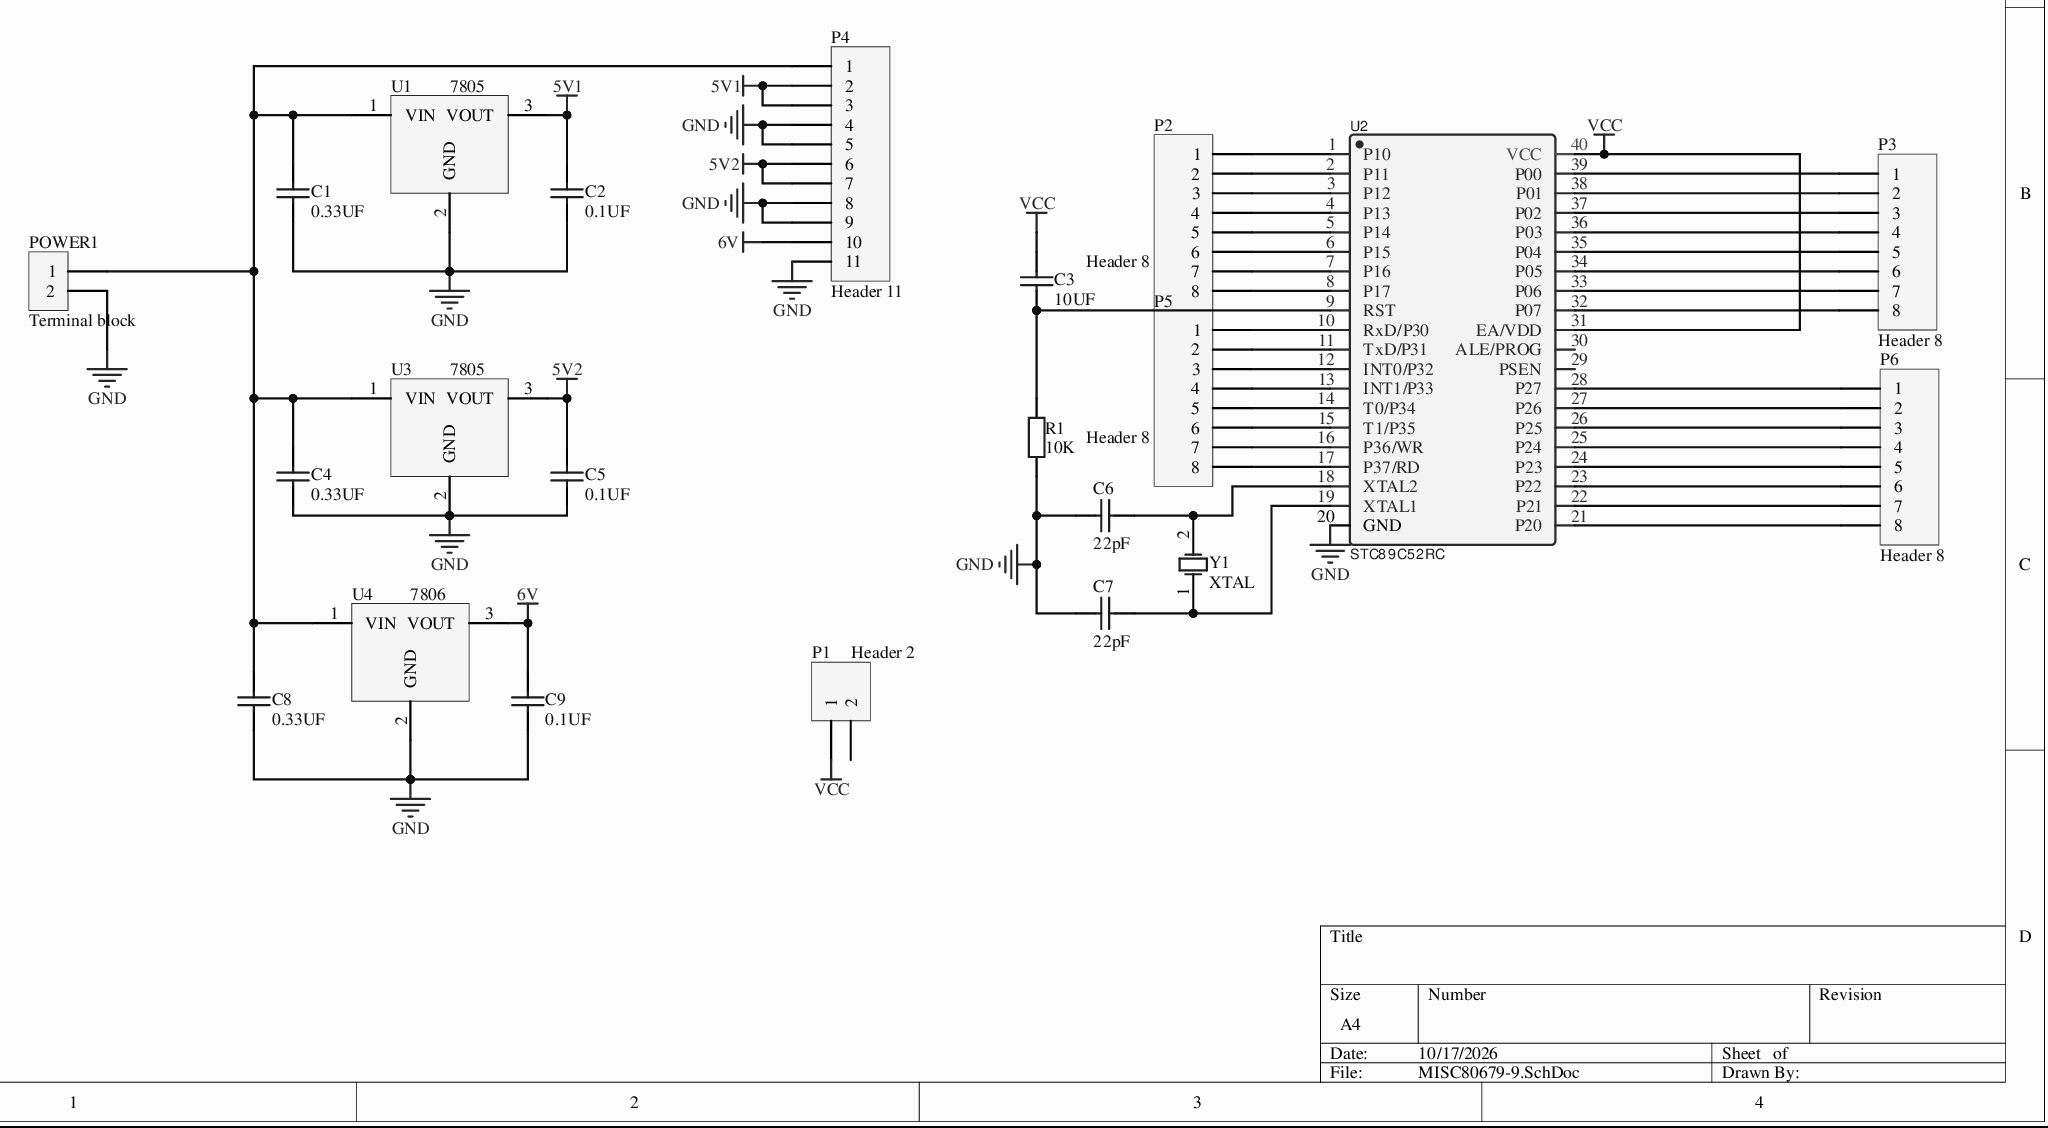
[diagram p0: MISC80679-9.SchDoc]
# Altium project MISC80679-3.PrjPcb
1 sheet, 22 parts. Net scope: global (net labels, ports and power ports of the same name join across sheets).
Board file: MISC80679.PcbDoc

## Sheet MISC80679-9.SchDoc
size A4

### Parts
C1  0.33UF  [CC 1.8*3.6]
C2  0.1UF  [CC 1.8*3.6]
C3  10UF  [CAP 1.5*4*8]
C4  0.33UF  [CC 1.8*3.6]
C5  0.1UF  [CC 1.8*3.6]
C6  22pF  [CC 1.8*3.6]
C7  22pF  [CC 1.8*3.6]
C8  0.33UF  [CC 1.8*3.6]
C9  0.1UF  [CC 1.8*3.6]
P1  Header 2  [HDR1X2]
P2  Header 8  [HDR1X8]
P3  Header 8  [HDR1X8]
P4  Header 11  [HDR1X11]
P5  Header 8  [HDR1X8]
P6  Header 8  [HDR1X8]
POWER1  Terminal block  [VH3.96-2A]
R1  10K  [AXIAL-0.4]
U1  7805  [TO220A]
U2  STC89C52RC  [STC89C52RC]
U3  7805  [TO220A]
U4  7806  [TO220A]
Y1  XTAL  [R38]

### Nets
5V1: C2.1 P4.2 P4.3 U1.3(VOUT)
5V2: C5.1 P4.6 P4.7 U3.3(VOUT)
6V: C9.1 P4.10 U4.3(VOUT)
GND: C1.2 C2.2 C4.2 C5.2 C6.2 C7.2 C8.2 C9.2 P4.4 P4.5 P4.8 P4.9 P4.11 POWER1.2 R1.1 U1.2(GND) U2.20(GND) U3.2(GND) U4.2(GND)
VCC: C3.1 P1.1 U2.31(EA/VDD) U2.40(VCC)
NetC1_1: C1.1 C4.1 C8.1 P4.1 POWER1.1 U1.1(VIN) U3.1(VIN) U4.1(VIN)
NetC3_2: C3.2 R1.2 U2.9(RST)
NetC6_1: C6.1 U2.18(XTAL2) Y1.2(OSC2)
NetC7_1: C7.1 U2.19(XTAL1) Y1.1(OSC1)
NetP2_1: P2.1 U2.1(P10)
NetP2_2: P2.2 U2.2(P11)
NetP2_3: P2.3 U2.3(P12)
NetP2_4: P2.4 U2.4(P13)
NetP2_5: P2.5 U2.5(P14)
NetP2_6: P2.6 U2.6(P15)
NetP2_7: P2.7 U2.7(P16)
NetP2_8: P2.8 U2.8(P17)
NetP3_1: P3.1 U2.39(P00)
NetP3_2: P3.2 U2.38(P01)
NetP3_3: P3.3 U2.37(P02)
NetP3_4: P3.4 U2.36(P03)
NetP3_5: P3.5 U2.35(P04)
NetP3_6: P3.6 U2.34(P05)
NetP3_7: P3.7 U2.33(P06)
NetP3_8: P3.8 U2.32(P07)
NetP5_1: P5.1 U2.10(RxD/P30)
NetP5_2: P5.2 U2.11(TxD/P31)
NetP5_3: P5.3 U2.12(INT0/P32)
NetP5_4: P5.4 U2.13(INT1/P33)
NetP5_5: P5.5 U2.14(T0/P34)
NetP5_6: P5.6 U2.15(T1/P35)
NetP5_7: P5.7 U2.16(P36/WR)
NetP5_8: P5.8 U2.17(P37/RD)
NetP6_1: P6.1 U2.28(P27)
NetP6_2: P6.2 U2.27(P26)
NetP6_3: P6.3 U2.26(P25)
NetP6_4: P6.4 U2.25(P24)
NetP6_5: P6.5 U2.24(P23)
NetP6_6: P6.6 U2.23(P22)
NetP6_7: P6.7 U2.22(P21)
NetP6_8: P6.8 U2.21(P20)

Not connected (* = marked no-connect by the designer): P1 2; U2 29(PSEN) 30(ALE/PROG)

### Library data of the parts
C1-C9 = Cap: Capacitor; Value: 100pF; Published: 8-Jun-2000; LatestRevisionDate: 17-Jul-2002; LatestRevisionNote: Re-released for DXP Platform.; PackageReference: RAD-0.3; PackageDescription: Radial Cap, Thru-Hole; 2 Leads; 0.3 in Pin Spacing; Publisher: Altium Limited
P1 = Header 2: Header, 2-Pin; LatestRevisionDate: 17-Jul-2002; LatestRevisionNote: Re-released for DXP Platform.; Publisher: Altium Limited
P2 P3 P5 P6 = Header 8: Header, 8-Pin; LatestRevisionDate: 17-Jul-2002; LatestRevisionNote: Re-released for DXP Platform.; Publisher: Altium Limited
P4 = Header 11: Header, 11-Pin; LatestRevisionDate: 17-Jul-2002; LatestRevisionNote: Re-released for DXP Platform.; Publisher: Altium Limited
POWER1 = VH2
R1 = Res2: Resistor; Value: 1K; Published: 8-Jun-2000; LatestRevisionDate: 17-Jul-2002; LatestRevisionNote: Re-released for DXP Platform.; PackageReference: AXIAL-0.4; PackageDescription: Axial Device, Thru-Hole; 2 Leads; 0.4 in Pin Spacing; Publisher: Altium Limited
U1 U3 U4 = LM7805
Y1 = XTAL: Crystal Oscillator; Published: 8-Jun-2000; LatestRevisionDate: 17-Jul-2002; LatestRevisionNote: Re-released for DXP Platform.; PackageReference: R38; PackageDescription: Crystal, Thru-Hole; 2 Leads; Body 3.1 x 8.2 mm (Dia.xH); Publisher: Altium Limited